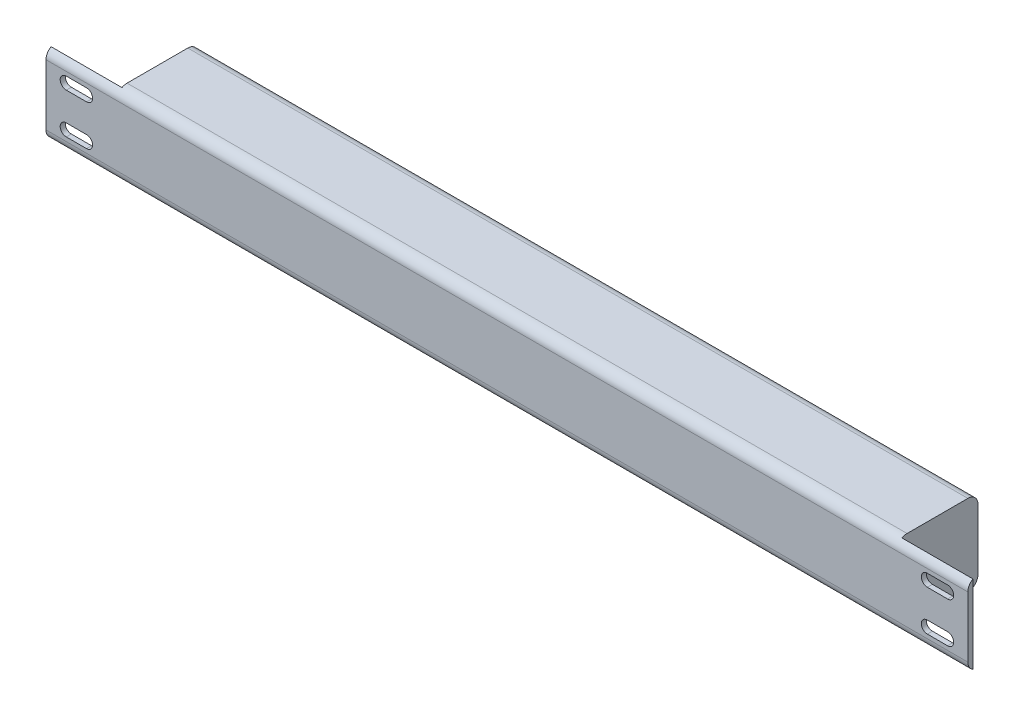
SolidWorks part; units mm, degrees
ref_plane "Front Plane" through (0, 0, 0) normal (0, 0, 1) x (1, 0, 0)
ref_plane "Top Plane" through (0, 0, 0) normal (0, 1, 0) x (1, 0, 0)
ref_plane "Right Plane" through (0, 0, 0) normal (1, 0, 0) x (0, 0, -1)
ref_plane "Plane4" through (0, 30, 0) normal (0, 1, 0) x (1, 0, 0)
sketch "Sketch1" plane through (0, 30, 0) normal (0, 1, 0) x (1, 0, 0)
  line L0 (-156.6667, 40) -> (-156.6667, -40)
  line L1 (-156.6667, -40) -> (613.3333, -40)
  line L2 (613.3333, -40) -> (613.3333, 40)
  line L3 (613.3333, 40) -> (-156.6667, 40)
  dimension "D1" = 80
  dimension "D2" = 770
extrude "Boss-Extrude1" add sketch "Sketch1" against normal blind 80
sketch "Sketch3" plane through (-156.6667, 0, 0) normal (-1, 0, 0) x (0, 0, 1)
  line L0 (35, -50) -> (35, 30)
  line L1 (35, 30) -> (40, 30)
  line L2 (40, 30) -> (40, -50)
  line L3 (40, -50) -> (35, -50)
  line L4 (40, -50) -> (40, 30) construction
  line L5 (-40, -50) -> (40, -50) construction
  line L6 (-40, 30) -> (40, 30) construction
  dimension "D1" = 0
  dimension "D2" = 0
  dimension "D3" = 0
extrude "Boss-Extrude2" add sketch "Sketch3" along normal blind 70
sketch "Sketch4" plane through (613.3333, 0, 0) normal (1, 0, 0) x (0, 0, -1)
  line L0 (-40, -50) -> (-40, 30)
  line L1 (-40, 30) -> (-35, 30)
  line L2 (-35, 30) -> (-35, -50)
  line L3 (-35, -50) -> (-40, -50)
  line L4 (-40, -50) -> (-40, 30) construction
  line L5 (-40, -50) -> (40, -50) construction
  dimension "D1" = 0
  dimension "D2" = 0
extrude "Boss-Extrude3" add sketch "Sketch4" along normal blind 70
sketch "Sketch6" plane through (0, 0, 40) normal (0, 0, 1) x (1, 0, 0)
  line L0 (-206.6667, -30) -> (-186.6667, -30) construction
  line L1 (-206.6667, -24) -> (-186.6667, -24)
  line L2 (228.3333, -1050) -> (228.3333, 48950) construction
  line L4 (-206.6667, -36) -> (-186.6667, -36)
  line L5 (-206.6667, 10) -> (-186.6667, 10) construction
  line L6 (-206.6667, 16) -> (-186.6667, 16)
  line L7 (-206.6667, 4) -> (-186.6667, 4)
  line L8 (663.3333, 10) -> (643.3333, 10) construction
  line L9 (-226.6667, 30) -> (683.3333, 30) construction
  line L10 (-226.6667, -50) -> (-226.6667, 30) construction
  line L11 (-226.6667, -50) -> (683.3333, -50) construction
  line L12 (663.3333, 16) -> (643.3333, 16)
  line L13 (663.3333, 4) -> (643.3333, 4)
  line L14 (663.3333, -30) -> (643.3333, -30) construction
  line L15 (663.3333, -24) -> (643.3333, -24)
  line L16 (663.3333, -36) -> (643.3333, -36)
  arc A0 (-206.6667, -24) -> (-206.6667, -36) centre (-206.6667, -30) ccw
  arc A1 (-206.6667, 16) -> (-206.6667, 4) centre (-206.6667, 10) ccw
  arc A2 (-186.6667, -36) -> (-186.6667, -24) centre (-186.6667, -30) ccw
  arc A3 (-186.6667, 4) -> (-186.6667, 16) centre (-186.6667, 10) ccw
  arc A4 (663.3333, 16) -> (663.3333, 4) centre (663.3333, 10) cw
  arc A5 (643.3333, 4) -> (643.3333, 16) centre (643.3333, 10) cw
  arc A6 (663.3333, -24) -> (663.3333, -36) centre (663.3333, -30) cw
  arc A7 (643.3333, -36) -> (643.3333, -24) centre (643.3333, -30) cw
  point P0 (-196.6667, -30)
  point P13 (-196.6667, 10)
  point P26 (228.3333, -50)
  point P28 (653.3333, 10)
  point P35 (653.3333, -30)
  dimension "D3" = 6
  dimension "D5" = 6
  dimension "D1" = 20
  dimension "D2" = 20
  dimension "D4" = 20
  dimension "D6" = 20
  dimension "D7" = 20
fillet "Fillet2" radius 10 4 edges at (228.3333, 30, 40) (228.3333, -50, 40) (228.3333, -50, -40) (228.3333, 30, -40)
extrude "Cut-Extrude1" cut sketch "Sketch6" against normal through all
